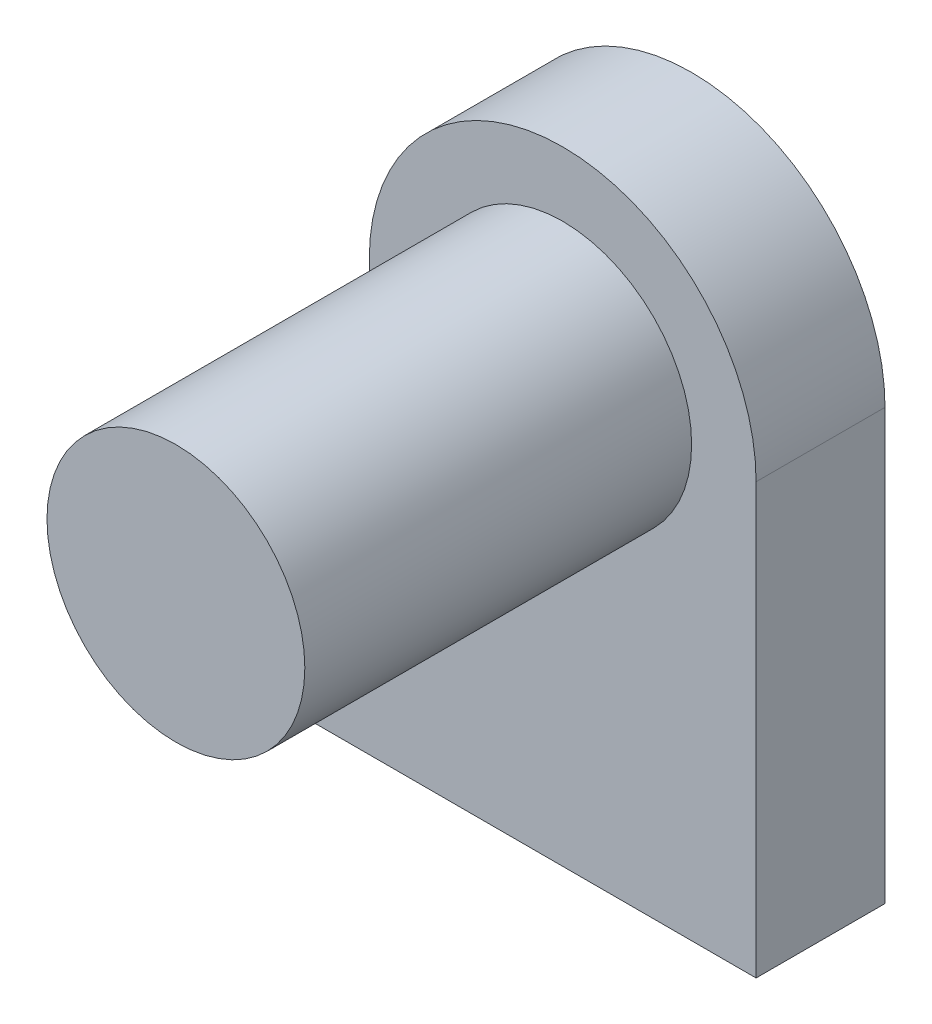
from build123d import *

# Parameters (mm, degrees)
SKETCH2_W           = 150
SKETCH2_H           = 25
BOSS_EXTRUDE1_DEPTH = 15
SKETCH3_R           = 30
BOSS_EXTRUDE2_DEPTH = 30
SKETCH4_R           = 5.5
CUT_EXTRUDE1_DEPTH  = 30
BOSS_EXTRUDE3_START = -120
SKETCH5_R           = 30
BOSS_EXTRUDE3_DEPTH = 120


with BuildPart() as part:
    # Sketch2 → Boss-Extrude1 (new, symmetric)
    with BuildSketch(Plane.XY):
        Rectangle(SKETCH2_W, SKETCH2_H)
    extrude(amount=BOSS_EXTRUDE1_DEPTH, both=True)

    # Sketch3 → Boss-Extrude2 (add)
    with BuildSketch(Plane.XY.offset(15)):
        with BuildLine():
            Line((-15, 87.5), (-15, 0))
            Line((-15, 0), (75, 0))
            Line((75, 0), (75, 87.5))
            ThreePointArc((75, 87.5), (30, 132.5), (-15, 87.5))
        make_face()
        with Locations((30, 87.5)):
            Circle(SKETCH3_R, mode=Mode.SUBTRACT)
    extrude(amount=-BOSS_EXTRUDE2_DEPTH)

    # Sketch4 → Cut-Extrude1 (cut)
    with BuildSketch(Plane(origin=(0, 12.5, 0), x_dir=(1, 0, 0), z_dir=(0, 1, 0))):
        with Locations(Location((-60, 0, 0), (0, 0, 270))):
            Circle(SKETCH4_R)
        with Locations(Location((-40, 0, 0), (0, 0, 270))):
            Circle(SKETCH4_R)
    extrude(amount=-CUT_EXTRUDE1_DEPTH, mode=Mode.SUBTRACT)

    # Sketch5 → Boss-Extrude3 (add)
    with BuildSketch(Plane(origin=(0, 0, -15), x_dir=(-1, 0, 0), z_dir=(0, 0, -1)).offset(BOSS_EXTRUDE3_START)):
        with Locations((-30, 87.5)):
            Circle(SKETCH5_R)
    extrude(amount=BOSS_EXTRUDE3_DEPTH)


solid = part.part
